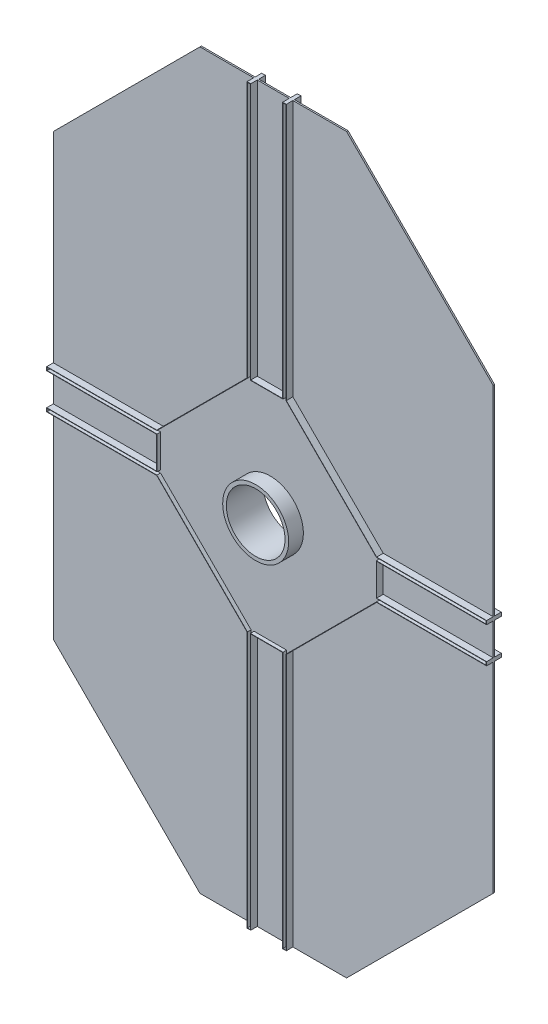
SolidWorks part; units mm, degrees
ref_plane "Front Plane" through (0, 0, 0) normal (0, 0, 1) x (1, 0, 0)
ref_plane "Top Plane" through (0, 0, 0) normal (0, 1, 0) x (1, 0, 0)
ref_plane "Right Plane" through (0, 0, 0) normal (1, 0, 0) x (0, 0, -1)
other "Configuration Table"
sketch "Sketch1" plane through (0, 0, 0) normal (0, 0, 1) x (1, 0, 0)
  circle A0 centre (-599.8842, -90) radius 40
  circle A1 centre (-599.8842, -90) radius 45
extrude "Boss-Extrude1" add sketch "Sketch1" along normal blind 50
ref_plane "Plane1" through (0, 0, 30) normal (0, 0, -1) x (-1, 0, 0)
sketch "Sketch4" plane through (0, 0, 30) normal (0, 0, -1) x (-1, 0, 0)
  line L1 (626.6609, -240) -> (749.8842, -116.7767)
  line L2 (749.8842, -63.2233) -> (626.6609, 60)
  line L3 (573.1075, 60) -> (449.8842, -63.2233)
  line L4 (449.8842, -116.7767) -> (573.1075, -240)
  line L5 (573.1075, 60) -> (626.6609, 60)
  line L6 (449.8842, -63.2233) -> (449.8842, -116.7767)
  line L7 (573.1075, -240) -> (626.6609, -240)
  line L8 (749.8842, -63.2233) -> (749.8842, -116.7767)
  line L9 (511.4958, -1.6117) -> (688.2725, -178.3883) construction
  line L10 (511.4958, -178.3883) -> (688.2725, -1.6117) construction
  circle A0 centre (599.8842, -90) radius 45
  circle A1 centre (599.8842, -90) radius 125 construction
  dimension "D2" = 250
extrude "Boss-Extrude2" add sketch "Sketch4" along normal blind 10
sketch "Sketch6" plane through (0, 0, 20) normal (0, 0, -1) x (-1, 0, 0)
  line L0 (899.8842, -390) -> (699.8842, -590)
  line L1 (899.8842, 210) -> (299.8842, 210)
  line L2 (899.8842, 210) -> (899.8842, -390)
  line L3 (899.8842, -390) -> (299.8842, -390)
  line L4 (299.8842, 210) -> (299.8842, -390)
  line L5 (899.8842, 210) -> (299.8842, -390) construction
  line L6 (899.8842, -390) -> (299.8842, 210) construction
  line L7 (499.8842, 410) -> (699.8842, 410)
  line L8 (499.8842, 410) -> (499.8842, -590)
  line L9 (499.8842, -590) -> (699.8842, -590)
  line L10 (699.8842, 410) -> (699.8842, -590)
  line L11 (499.8842, 410) -> (699.8842, -590) construction
  line L12 (499.8842, -590) -> (699.8842, 410) construction
  line L13 (499.8842, -590) -> (299.8842, -390)
  line L14 (299.8842, 210) -> (499.8842, 410)
  line L15 (699.8842, 410) -> (899.8842, 210)
  circle A0 centre (599.8842, -90) radius 40
  point P0 (599.8842, -90)
  point P6 (599.8842, -90)
  line M4 (626.6609, 60) -> (573.1075, 60)
  line M5 (573.1075, 60) -> (449.8842, -63.2233)
  line M6 (449.8842, -63.2233) -> (449.8842, -116.7767)
  line M7 (449.8842, -116.7767) -> (573.1075, -240)
  line M8 (573.1075, -240) -> (626.6609, -240)
  line M9 (626.6609, -240) -> (749.8842, -116.7767)
  line M10 (749.8842, -116.7767) -> (749.8842, -63.2233)
  line M11 (749.8842, -63.2233) -> (626.6609, 60)
  circle M12 centre (599.8842, -90) radius 45
  dimension "D1" = 600
  dimension "D3" = 1000
extrude "Boss-Extrude3" add sketch "Sketch6" against normal blind 2 from offset 4 contours L10 L1 L8 M5 M4 M11 | L10 L7 L8 L1 | L14 L1 L8 | L8 L1 L4 M5 | L8 M5 M6 M7 | L8 L4 L3 M7 | L10 L8 L3 M9 M8 M7 | L10 L3 L8 L9 | L13 L8 L3 | L3 L10 L0 | L10 L3 L2 M9 | L10 M11 M9 M10 | L1 L10 L2 M11 | L15 L10 L1 | L10 L8 M11 M4 M5 M7 M8 M9 M12 offset against normal yes
sketch "Sketch7" plane through (0, 0, 20) normal (0, 0, -1) x (-1, 0, 0)
  line L0 (899.8842, 210) -> (899.8842, -390) construction
  line L1 (749.8842, -63.2233) -> (899.8842, -63.2233)
  line L2 (749.8842, -63.2233) -> (749.8842, -68.2233)
  line L3 (749.8842, -68.2233) -> (899.8842, -68.2233)
  line L4 (899.8842, -63.2233) -> (899.8842, -68.2233)
  line L5 (749.8842, -111.7767) -> (899.8842, -111.7767)
  line L6 (749.8842, -111.7767) -> (749.8842, -116.7767)
  line L7 (749.8842, -116.7767) -> (899.8842, -116.7767)
  line L8 (899.8842, -111.7767) -> (899.8842, -116.7767)
  line L9 (749.8842, -116.7767) -> (749.8842, -63.2233) construction
  line L10 (599.8842, -50) -> (599.8842, -130) construction
  line L11 (299.8842, -111.7767) -> (299.8842, -116.7767)
  line L12 (449.8842, -116.7767) -> (299.8842, -116.7767)
  line L13 (449.8842, -111.7767) -> (449.8842, -116.7767)
  line L14 (449.8842, -111.7767) -> (299.8842, -111.7767)
  line L15 (299.8842, -63.2233) -> (299.8842, -68.2233)
  line L16 (449.8842, -68.2233) -> (299.8842, -68.2233)
  line L17 (449.8842, -63.2233) -> (449.8842, -68.2233)
  line L18 (449.8842, -63.2233) -> (299.8842, -63.2233)
  line L19 (499.8842, -590) -> (699.8842, -590) construction
  line L20 (626.6609, -240) -> (621.6609, -240)
  line L21 (626.6609, -240) -> (626.6609, -590)
  line L22 (626.6609, -590) -> (621.6609, -590)
  line L23 (621.6609, -240) -> (621.6609, -590)
  line L24 (578.1075, -240) -> (573.1075, -240)
  line L25 (578.1075, -240) -> (578.1075, -590)
  line L26 (578.1075, -590) -> (573.1075, -590)
  line L27 (573.1075, -240) -> (573.1075, -590)
  line L28 (639.8842, -90) -> (559.8842, -90) construction
  line L29 (573.1075, 60) -> (573.1075, 410)
  line L30 (578.1075, 410) -> (573.1075, 410)
  line L31 (578.1075, 60) -> (578.1075, 410)
  line L32 (578.1075, 60) -> (573.1075, 60)
  line L33 (621.6609, 60) -> (621.6609, 410)
  line L34 (626.6609, 410) -> (621.6609, 410)
  line L35 (626.6609, 60) -> (626.6609, 410)
  line L36 (626.6609, 60) -> (621.6609, 60)
  circle A0 centre (599.8842, -90) radius 40 construction
  dimension "D1" = 5
  dimension "D2" = 5
  dimension "D3" = 5
  dimension "D4" = 5
extrude "Boss-Extrude4" add sketch "Sketch7" against normal blind 10
sketch "Sketch8" plane through (0, 0, 20) normal (0, 0, -1) x (-1, 0, 0)
  line L32 (749.8842, -63.2233) -> (626.6609, 60)
  line L33 (626.6609, 60) -> (626.6609, 410)
  line L34 (626.6609, 410) -> (621.6609, 410)
  line L35 (621.6609, 410) -> (621.6609, 60)
  line L36 (621.6609, 60) -> (578.1075, 60)
  line L37 (578.1075, 60) -> (578.1075, 410)
  line L38 (578.1075, 410) -> (573.1075, 410)
  line L39 (573.1075, 410) -> (573.1075, 60)
  line L40 (573.1075, 60) -> (449.8842, -63.2233)
  line L41 (449.8842, -63.2233) -> (299.8842, -63.2233)
  line L42 (299.8842, -63.2233) -> (299.8842, -68.2233)
  line L43 (299.8842, -68.2233) -> (449.8842, -68.2233)
  line L44 (449.8842, -68.2233) -> (449.8842, -111.7767)
  line L45 (449.8842, -111.7767) -> (299.8842, -111.7767)
  line L46 (299.8842, -111.7767) -> (299.8842, -116.7767)
  line L47 (299.8842, -116.7767) -> (449.8842, -116.7767)
  line L48 (449.8842, -116.7767) -> (573.1075, -240)
  line L49 (573.1075, -240) -> (573.1075, -590)
  line L50 (573.1075, -590) -> (578.1075, -590)
  line L51 (578.1075, -590) -> (578.1075, -240)
  line L52 (578.1075, -240) -> (621.6609, -240)
  line L53 (621.6609, -240) -> (621.6609, -590)
  line L54 (621.6609, -590) -> (626.6609, -590)
  line L55 (626.6609, -590) -> (626.6609, -240)
  line L56 (626.6609, -240) -> (749.8842, -116.7767)
  line L57 (749.8842, -116.7767) -> (899.8842, -116.7767)
  line L58 (899.8842, -116.7767) -> (899.8842, -111.7767)
  line L59 (899.8842, -111.7767) -> (749.8842, -111.7767)
  line L60 (749.8842, -111.7767) -> (749.8842, -68.2233)
  line L61 (749.8842, -68.2233) -> (899.8842, -68.2233)
  line L62 (899.8842, -68.2233) -> (899.8842, -63.2233)
  line L63 (899.8842, -63.2233) -> (749.8842, -63.2233)
  line L64 (749.8842, -63.2233) -> (626.6609, 60)
  line L65 (626.6609, 60) -> (626.6609, 410)
  line L66 (626.6609, 410) -> (621.6609, 410)
  line L67 (621.6609, 410) -> (621.6609, 60)
  line L68 (621.6609, 60) -> (578.1075, 60)
  line L69 (578.1075, 60) -> (578.1075, 410)
  line L70 (578.1075, 410) -> (573.1075, 410)
  line L71 (573.1075, 410) -> (573.1075, 60)
  line L72 (573.1075, 60) -> (449.8842, -63.2233)
  line L73 (449.8842, -63.2233) -> (299.8842, -63.2233)
  line L74 (299.8842, -63.2233) -> (299.8842, -68.2233)
  line L75 (299.8842, -68.2233) -> (449.8842, -68.2233)
  line L76 (449.8842, -68.2233) -> (449.8842, -111.7767)
  line L77 (449.8842, -111.7767) -> (299.8842, -111.7767)
  line L78 (299.8842, -111.7767) -> (299.8842, -116.7767)
  line L79 (299.8842, -116.7767) -> (449.8842, -116.7767)
  line L80 (449.8842, -116.7767) -> (573.1075, -240)
  line L81 (573.1075, -240) -> (573.1075, -590)
  line L82 (573.1075, -590) -> (578.1075, -590)
  line L83 (578.1075, -590) -> (578.1075, -240)
  line L84 (578.1075, -240) -> (621.6609, -240)
  line L85 (621.6609, -240) -> (621.6609, -590)
  line L86 (621.6609, -590) -> (626.6609, -590)
  line L87 (626.6609, -590) -> (626.6609, -240)
  line L88 (626.6609, -240) -> (749.8842, -116.7767)
  line L89 (749.8842, -116.7767) -> (899.8842, -116.7767)
  line L90 (899.8842, -116.7767) -> (899.8842, -111.7767)
  line L91 (899.8842, -111.7767) -> (749.8842, -111.7767)
  line L92 (749.8842, -111.7767) -> (749.8842, -68.2233)
  line L93 (749.8842, -68.2233) -> (899.8842, -68.2233)
  line L94 (899.8842, -68.2233) -> (899.8842, -63.2233)
  line L95 (899.8842, -63.2233) -> (749.8842, -63.2233)
  dimension "D1" = 0
extrude "Extrude-Thin2" add sketch "Sketch8" along normal blind 5 and the other way blind 15 thin thin type one direction reverse wall 0.5
